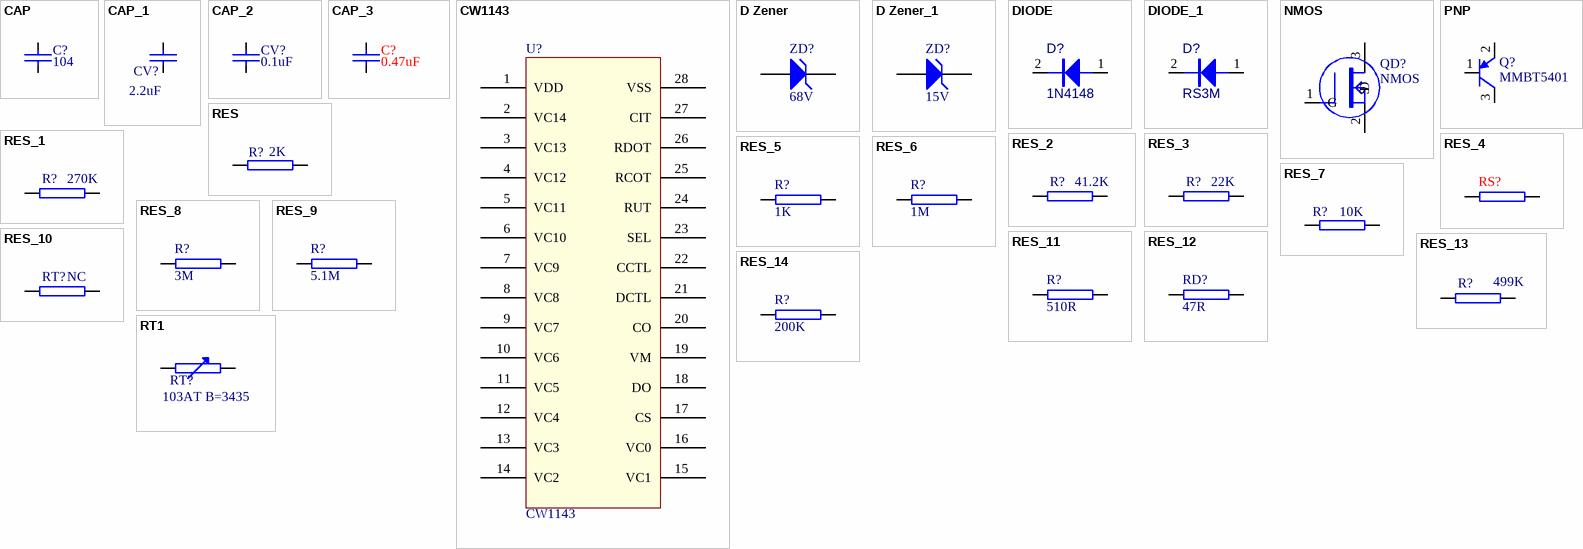
[diagram p0: symbols CAP to RT1]
# Altium schematic symbol library MISC84297-4.SchLib: 27 symbols
Pins are listed as number, name and electrical type; pins without a type are passive.


## CAP
designator C?, comment 104
footprint 0603
footprint 0603C
footprint CAP0603 (CAP0402)
pins: 1, 2

## CAP_1
designator CV?, comment 2.2uF
footprint 0805C
footprint CAP0603 (CAP0402)
footprint CAP0805
pins: 1, 2

## CAP_2
designator CV?, comment 0.1uF
footprint 0603C
footprint CAP0603
pins: 1, 2

## CAP_3
designator C?, comment 0.47uF
footprint 0603C
footprint CAP0603 (CAP0402)
pins: 1, 2

## CW1143
designator U?
footprint SSOP-28-0.635 (Footprint not found)
pins: 1 VDD, 2 VC14, 3 VC13, 4 VC12, 5 VC11, 6 VC10, 7 VC9, 8 VC8, 9 VC7, 10 VC6, 11 VC5, 12 VC4, 13 VC3, 14 VC2, 15 VC1, 16 VC0, 17 CS, 18 DO, 19 VM, 20 CO, 21 DCTL, 22 CCTL, 23 SEL, 24 RUT, 25 RCOT, 26 RDOT, 27 CIT, 28 VSS

## D Zener
designator ZD?, comment 68V
Zener Diode
footprint SOD123
simulation model ZENER (Diode)
signal-integrity model D Zener
pins: 1 A, 2 K

## D Zener_1
designator ZD?, comment 15V
Zener Diode
footprint SOD323
simulation model ZENER (Diode)
signal-integrity model D Zener
pins: 1 A, 2 K

## DIODE
designator D?, comment 1N4148
DIODE
footprint DIODE0.4
footprint DIODE0.1
footprint DIODE0.3
footprint DIODE0.5
footprint SOD323
pins: 1 A, 2 K
2 alternate drawings of the same symbol

## DIODE_1
designator D?, comment RS3M
DIODE
footprint DIODE0.4
footprint DIODE0.1
footprint DIODE0.3
footprint DIODE0.5
footprint SMC
pins: 1 A, 2 K
2 alternate drawings of the same symbol

## NMOS
designator QD?
footprint SOT-23-3
footprint TO-252
footprint to-252-A
footprint TO-252-A
footprint TO-252-A
footprint TOLL
footprint TO-263
footprint TO-263-TOLL
footprint TOLL_123 (SMD MOS)
pins: 1 G, 2 S, 3 D

## PNP
designator Q?, comment MMBT5401
PNP Bipolar Transistor
footprint SOT-23B_N (SOT23, 3-Leads, Body 2.9x1.3mm, Pitch 0.95mm, Lead Span 2.4mm, IPC Medium Density)
footprint SOT-23B_L (SOT23, 3-Leads, Body 2.9x1.3mm, Pitch 0.95mm, Lead Span 2.4mm, IPC High Density)
footprint SOT-23B_M (SOT23, 3-Leads, Body 2.9x1.3mm, Pitch 0.95mm, Lead Span 2.4mm, IPC Low Density)
simulation model PNP
signal-integrity model PNP
footprint SOT-23-3
pins: 1 B, 2 E, 3 C

## RES
designator R?, comment 2K
footprint 0603
footprint RES0805
pins: 1, 2

## RES_1
designator R?, comment 270K
footprint 0603
footprint 0603R
footprint RES0603
pins: 1, 2

## RES_2
designator R?, comment 41.2K
footprint 0603
footprint 0603R
footprint RES0603
pins: 1, 2

## RES_3
designator R?, comment 22K
footprint 0603
footprint 0603R
footprint RES0603
pins: 1, 2

## RES_4
designator RS?
footprint 0603
footprint 2512
pins: 1, 2

## RES_5
designator R?, comment 1K
footprint 0603
footprint 0603R
footprint RES0603
pins: 1, 2

## RES_6
designator R?, comment 1M
footprint 0603
footprint 0603R
footprint RES0603
pins: 1, 2

## RES_7
designator R?, comment 10K
footprint 0603
footprint 0603R
footprint RES0603
pins: 1, 2

## RES_8
designator R?, comment 3M
footprint 0603
footprint 0603R
footprint RES0603
pins: 1, 2

## RES_9
designator R?, comment 5.1M
footprint 0603
footprint 0603R
footprint RES0603
pins: 1, 2

## RES_10
designator RT?, comment NC
footprint 0603
footprint 0603R
footprint RES0603
pins: 1, 2

## RES_11
designator R?, comment 510R
footprint 0603
footprint 0603R
footprint RES0603
pins: 1, 2

## RES_12
designator RD?, comment 47R
footprint 0603
footprint 0603R
footprint RES0603
pins: 1, 2

## RES_13
designator R?, comment 499K
footprint 0603
footprint 0603R
footprint RES0603
pins: 1, 2

## RES_14
designator R?, comment 200K
footprint 0603
footprint 0603R
footprint RES0603
pins: 1, 2

## RT1
designator RT?, comment 103AT B=3435
footprint WK
pins: 1, 2